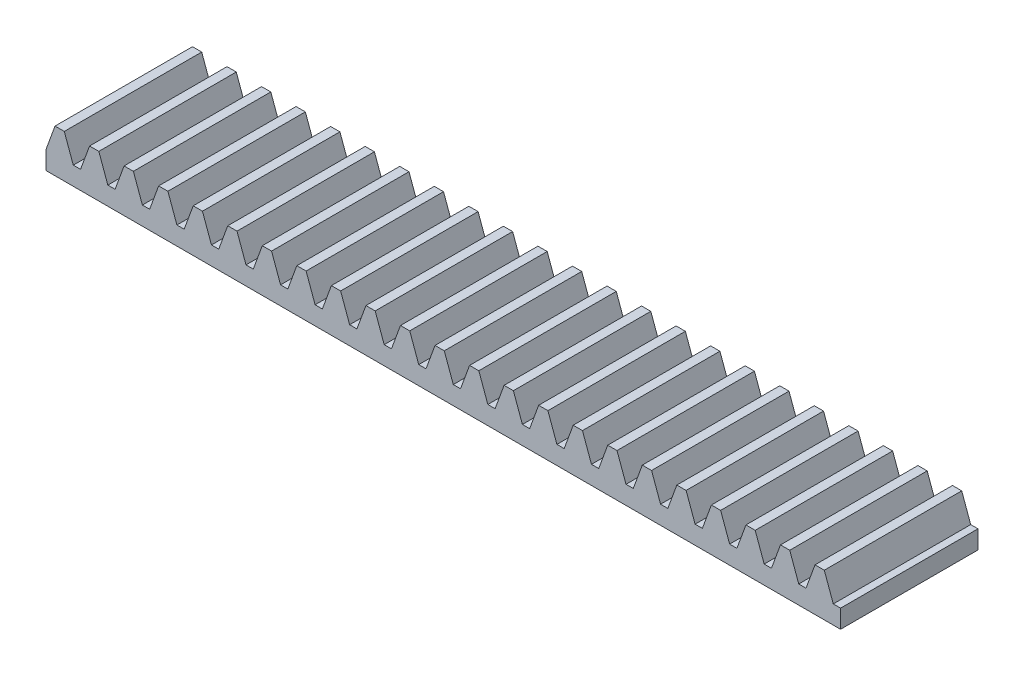
from build123d import *

# Parameters (mm, degrees)
SKETCH1_W           = 5
SKETCH1_H           = 5
BOSS_EXTRUDE1_DEPTH = 150
BOSS_EXTRUDE2_DEPTH = 150


with BuildPart() as part:
    # Sketch1 → Boss-Extrude1 (new body)
    with BuildSketch(Plane.XY):
        with Locations((2.5, 2.5)):
            Rectangle(SKETCH1_W, SKETCH1_H)
    extrude(amount=BOSS_EXTRUDE1_DEPTH)

    # Sketch2 → Boss-Extrude2 (add)
    with BuildSketch(Plane.XY):
        Polygon((0, 20), (9.827196325, 47), (19.941466624, 47), (29.76866295, 20), (37.699111843, 20), (47.526308168, 47), (57.640578467, 47), (67.467774793, 20), (75.398223686, 20), (85.225420011, 47), (95.33969031, 47), (105.166886636, 20), (113.097335529, 20), (122.924531854, 47), (133.038802154, 47), (142.865998479, 20), (150.796447372, 20), (160.623643697, 47), (170.737913997, 47), (180.565110322, 20), (188.495559215, 20), (198.322755541, 47), (208.43702584, 47), (218.264222165, 20), (226.194671058, 20), (236.021867384, 47), (246.136137683, 47), (255.963334008, 20), (263.893782902, 20), (273.720979227, 47), (283.835249526, 47), (293.662445851, 20), (301.592894745, 20), (311.42009107, 47), (321.534361369, 47), (331.361557694, 20), (339.292006588, 20), (349.119202913, 47), (359.233473212, 47), (369.060669537, 20), (376.991118431, 20), (386.818314756, 47), (396.932585055, 47), (406.75978138, 20), (414.690230274, 20), (424.517426599, 47), (434.631696898, 47), (444.458893223, 20), (452.389342117, 20), (462.216538442, 47), (472.330808741, 47), (482.158005066, 20), (490.08845396, 20), (499.915650285, 47), (510.029920584, 47), (519.85711691, 20), (527.787565803, 20), (537.614762128, 47), (547.729032427, 47), (557.556228753, 20), (565.486677646, 20), (575.313873971, 47), (585.42814427, 47), (595.255340596, 20), (603.185789489, 20), (613.012985814, 47), (623.127256114, 47), (632.954452439, 20), (640.884901332, 20), (650.712097658, 47), (660.826367957, 47), (670.653564282, 20), (678.584013175, 20), (688.411209501, 47), (698.5254798, 47), (708.352676125, 20), (716.283125018, 20), (726.110321344, 47), (736.224591643, 47), (746.051787968, 20), (753.982236862, 20), (763.809433187, 47), (773.923703486, 47), (783.750899811, 20), (791.681348705, 20), (801.50854503, 47), (811.622815329, 47), (821.450011654, 20), (829.380460548, 20), (839.207656873, 47), (849.321927172, 47), (859.149123497, 20), (867.079572391, 20), (867.079572391, 0), (0, 0), align=None)
    extrude(amount=BOSS_EXTRUDE2_DEPTH)


solid = part.part
